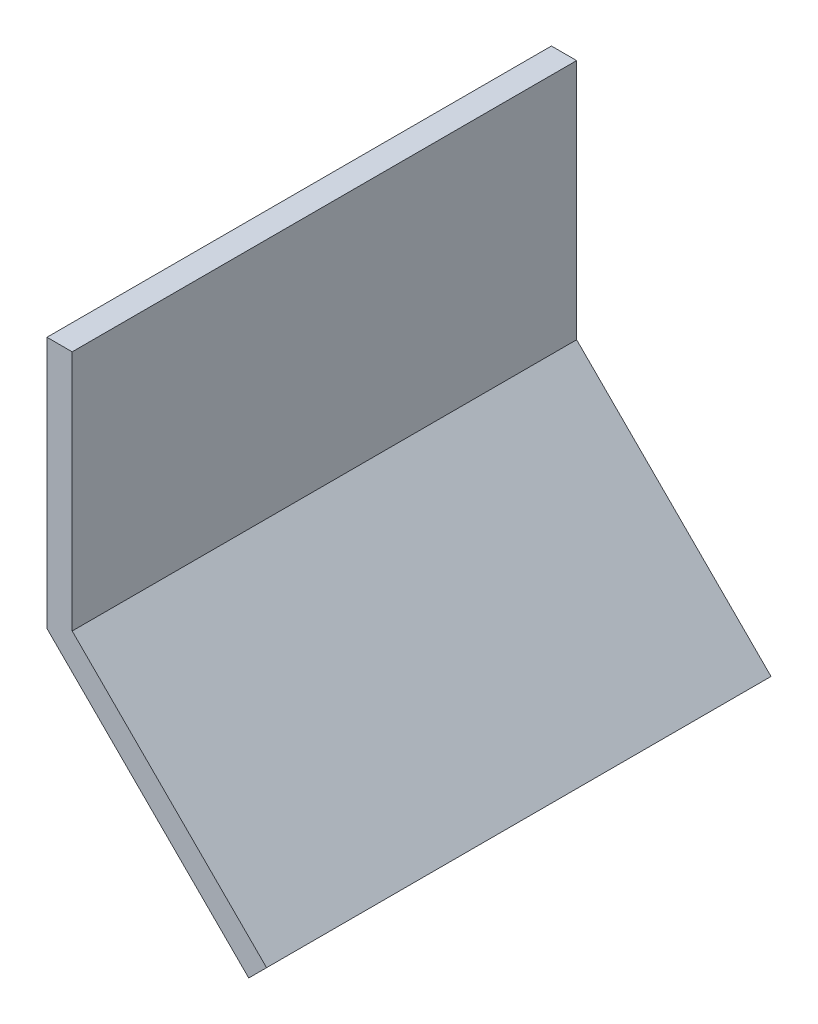
from build123d import *

# Parameters (mm, degrees)
EXTRUDE_2_DEPTH          = 100
CUT_EXTRUDE_1_DEPTH      = 140.946373206
CUT_EXTRUDE_1_DEPTH_BACK = 140.946373206
SKETCH_2_W               = 5
SKETCH_2_H               = 42.071067812
EXTRUDE_3_DEPTH          = 10


with BuildPart() as part:
    # 草图1 → 凸台-拉伸2 (new body)
    with BuildSketch(Plane.XY):
        Polygon((0, 0), (0, -50), (40, -90), (43.535533906, -86.464466094), (5, -47.928932188), (5, 0), align=None)
    extrude(amount=EXTRUDE_2_DEPTH)

    # 草图2 → 切除-拉伸1 (cut, two sides: drawn at the far end of the back side and taken through both)
    with BuildSketch(Plane(origin=(5, 0, 0), x_dir=(0, 0, -1), z_dir=(1, 0, 0)).offset(-CUT_EXTRUDE_1_DEPTH_BACK)):
        Polygon((0, 0), (-5, 0), (-5, -5), (-5, -42.928932188), (-5, -47.928932188), (0, -47.928932188), align=None)
        with Locations((-2.5, -68.964466094)):
            Rectangle(SKETCH_2_W, SKETCH_2_H)
        with Locations((-97.5, -68.964466094)):
            Rectangle(SKETCH_2_W, SKETCH_2_H)
        Polygon((-95, -5), (-95, 0), (-100, 0), (-100, -47.928932188), (-95, -47.928932188), (-95, -42.928932188), align=None)
    extrude(amount=CUT_EXTRUDE_1_DEPTH + CUT_EXTRUDE_1_DEPTH_BACK, mode=Mode.SUBTRACT)

    # 草图3 → 凸台-拉伸3 (add)
    with BuildSketch(Plane.XY.offset(95)):
        Polygon((0, -50), (40, -90), (43.535533906, -86.464466094), (5, -47.928932188), (5, 0), (0, 0), align=None)
    extrude(amount=EXTRUDE_3_DEPTH)


solid = part.part
